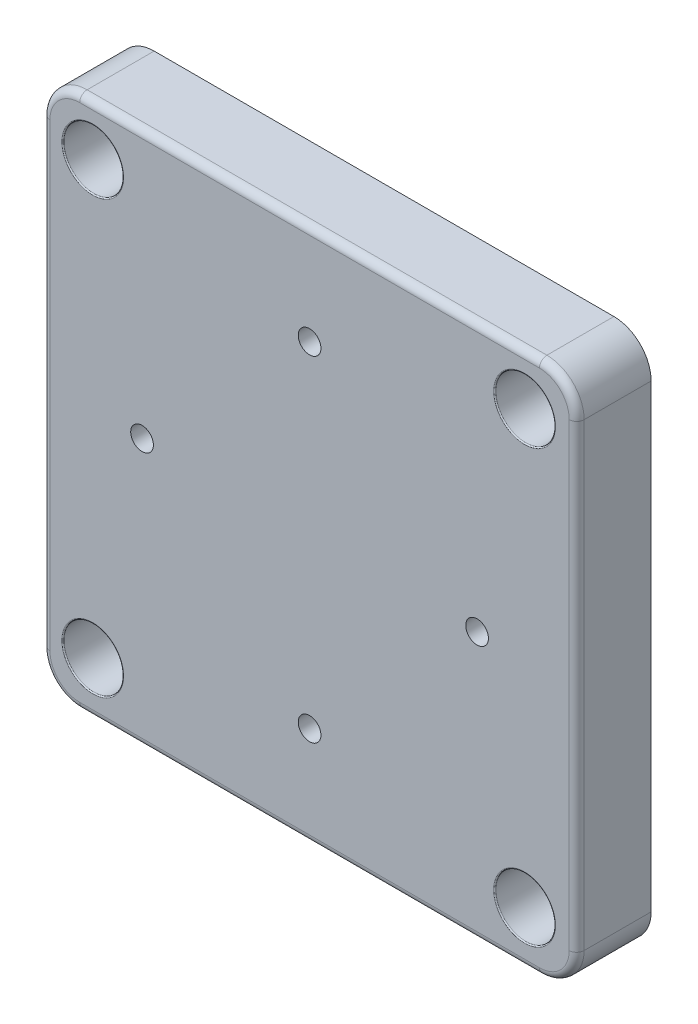
from build123d import *

# Parameters (mm, degrees)
SKETCH1_W           = 71.75
SKETCH1_H           = 71.75
SKETCH1_R           = 4
BOSS_EXTRUDE1_DEPTH = 10
FILLET1_R           = 5
FILLET2_R           = 1
FILLET4_R           = 0.15
SKETCH2_R           = 1.525
CUT_EXTRUDE1_DEPTH  = 10


with BuildPart() as part:
    # Sketch1 → Boss-Extrude1 (new body)
    with BuildSketch(Plane.XY):
        Rectangle(SKETCH1_W, SKETCH1_H)
        with Locations((-29.125, 29.125)):
            Circle(SKETCH1_R, mode=Mode.SUBTRACT)
        with Locations((28.875, 29.125)):
            Circle(SKETCH1_R, mode=Mode.SUBTRACT)
        with Locations((28.875, -28.875)):
            Circle(SKETCH1_R, mode=Mode.SUBTRACT)
        with Locations((-29.125, -28.875)):
            Circle(SKETCH1_R, mode=Mode.SUBTRACT)
    extrude(amount=BOSS_EXTRUDE1_DEPTH)

    # Fillet1
    fillet1_edges = [part.edges().sort_by_distance(p)[0] for p in [
        (-35.875, 35.875, 5),
        (35.875, 35.875, 5),
        (35.875, -35.875, 5),
        (-35.875, -35.875, 5),
    ]]
    fillet(fillet1_edges, radius=FILLET1_R)

    # Fillet2
    fillet2_edges = [part.edges().sort_by_distance(p)[0] for p in [
        (35.875, 0, 10),
        (0, -35.875, 10),
        (-35.875, 0, 10),
        (0, 35.875, 10),
        (-34.410533906, 34.410533906, 10),
        (34.410533906, 34.410533906, 10),
        (-34.410533906, -34.410533906, 10),
        (34.410533906, -34.410533906, 10),
    ]]
    fillet(fillet2_edges, radius=FILLET2_R)

    # Fillet4
    fillet4_edges = [part.edges().sort_by_distance(p)[0] for p in [
        (-33.125, 29.125, 10),
        (24.875, 29.125, 10),
        (24.875, -28.875, 10),
        (-33.125, -28.875, 10),
    ]]
    fillet(fillet4_edges, radius=FILLET4_R)

    # Sketch2 → Cut-Extrude1 (cut)
    with BuildSketch(Plane.XY.offset(10)):
        with Locations((0, 22.5)):
            Circle(SKETCH2_R)
        with Locations((22.5, 0)):
            Circle(SKETCH2_R)
        with Locations((0, -22.5)):
            Circle(SKETCH2_R)
        with Locations((-22.5, 0)):
            Circle(SKETCH2_R)
    extrude(amount=-CUT_EXTRUDE1_DEPTH, mode=Mode.SUBTRACT)


solid = part.part
